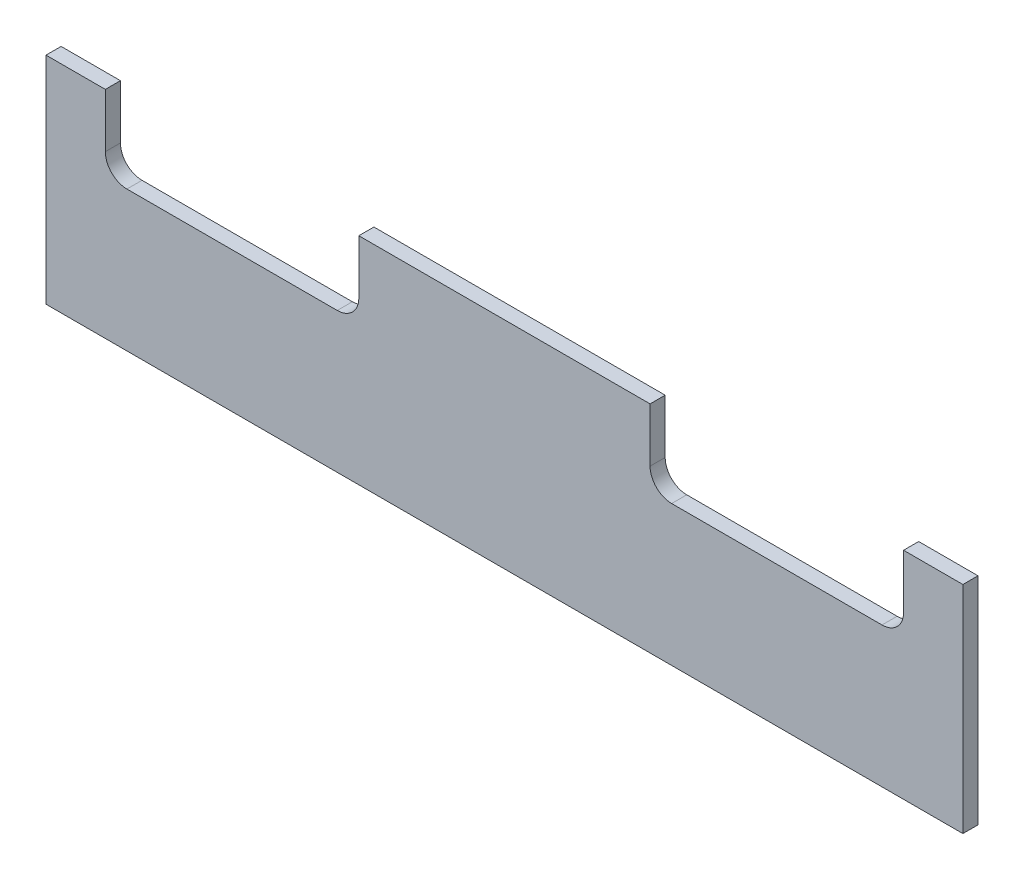
SolidWorks part; units mm, degrees
ref_plane "前视基准面" through (0, 0, 0) normal (0, 0, 1) x (1, 0, 0)
ref_plane "上视基准面" through (0, 0, 0) normal (0, 1, 0) x (1, 0, 0)
ref_plane "右视基准面" through (0, 0, 0) normal (1, 0, 0) x (0, 0, -1)
sketch "草图1" plane through (0, 0, 0) normal (0, 0, 1) x (1, 0, 0)
  line L1 (-425, -100) -> (425, -100)
  line L2 (-425, -100) -> (-425, 100)
  line L3 (-425, 100) -> (425, 100)
  line L4 (425, -100) -> (425, 100)
  line L5 (-425, -100) -> (425, 100) construction
  line L6 (-425, 100) -> (425, -100) construction
  point P0 (0, 0)
  dimension "D1" = 200
  dimension "D2" = 850
extrude "凸台-拉伸1" add sketch "草图1" along normal blind 14
sketch "草图2" plane through (0, 0, 0) normal (0, 0, -1) x (-1, 0, 0)
  line L0 (370, 100) -> (370, 30)
  line L1 (-425, 100) -> (425, 100) construction
  line L2 (370, 30) -> (135, 30)
  line L3 (135, 30) -> (135, 100)
  line L4 (135, 100) -> (370, 100)
  line L6 (0, -100) -> (0, 100) construction
  line L7 (425, -100) -> (-425, -100) construction
  line L8 (425, 100) -> (425, -100) construction
  line L9 (-135, 100) -> (-370, 100)
  line L10 (-135, 30) -> (-135, 100)
  line L11 (-370, 30) -> (-135, 30)
  line L12 (-370, 100) -> (-370, 30)
  dimension "D1" = 55
  dimension "D2" = 235
  dimension "D3" = 70
extrude "切除-拉伸1" cut sketch "草图2" against normal up to next
fillet "圆角1" radius 20 4 edges at (-370, 30, 7) (-135, 30, 7) (370, 30, 7) (135, 30, 7)
